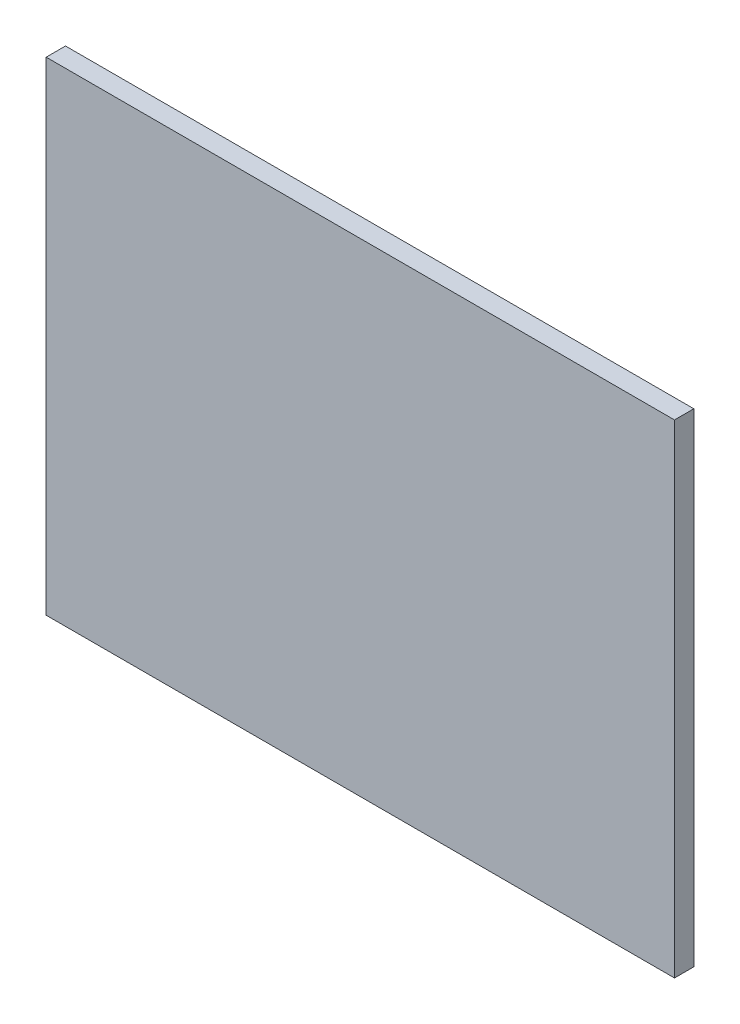
SolidWorks part; units mm, degrees
material "Q235"
ref_plane "Front Plane" through (0, 0, 0) normal (0, 0, 1) x (1, 0, 0)
ref_plane "Top Plane" through (0, 0, 0) normal (0, 1, 0) x (1, 0, 0)
ref_plane "Right Plane" through (0, 0, 0) normal (1, 0, 0) x (0, 0, -1)
sketch "Sketch1" plane through (0, 0, 0) normal (0, 0, 1) x (1, 0, 0)
  line L1 (0, 0) -> (390, 0)
  line L2 (0, 0) -> (0, -300)
  line L3 (0, -300) -> (390, -300)
  line L4 (390, 0) -> (390, -300)
  dimension "D1" = 390
  dimension "D2" = 300
extrude "Boss-Extrude1" add sketch "Sketch1" along normal blind 12
